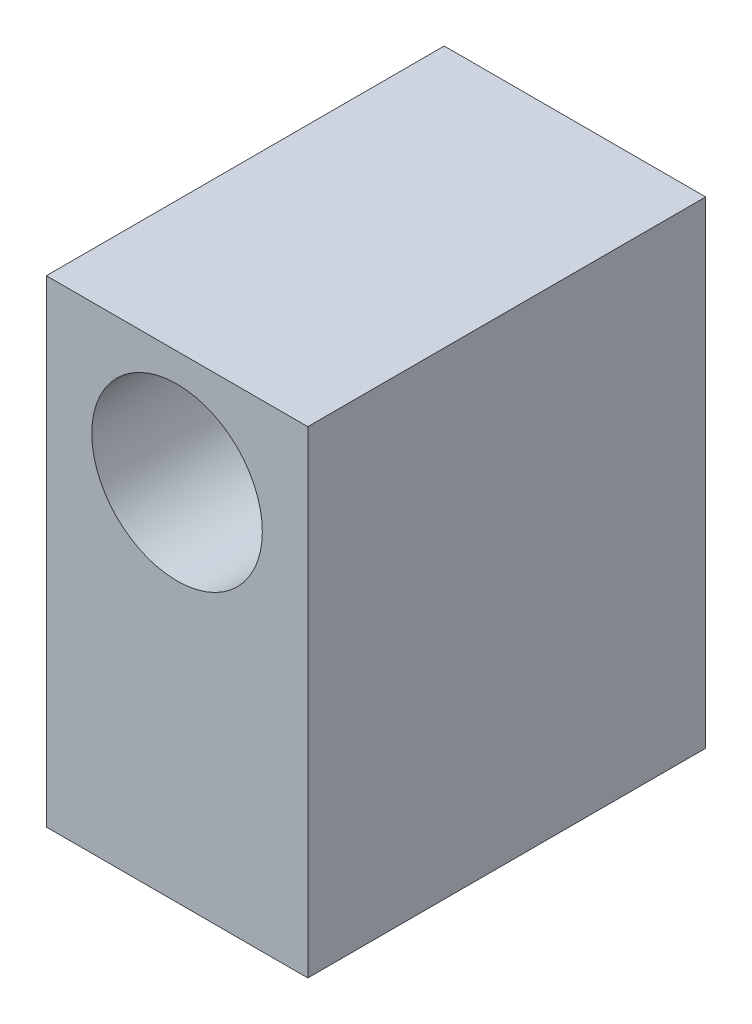
SolidWorks part; units mm, degrees
material "6061 合金"
ref_plane "前视基准面" through (0, 0, 0) normal (0, 0, 1) x (1, 0, 0)
ref_plane "上视基准面" through (0, 0, 0) normal (0, 1, 0) x (1, 0, 0)
ref_plane "右视基准面" through (0, 0, 0) normal (1, 0, 0) x (0, 0, -1)
sketch "草图1" plane through (0, 0, 0) normal (0, 0, 1) x (1, 0, 0)
  line L1 (-10.3871, 22.756) -> (12.6129, 22.756)
  line L2 (-10.3871, 22.756) -> (-10.3871, -19.244)
  line L3 (-10.3871, -19.244) -> (12.6129, -19.244)
  line L4 (12.6129, 22.756) -> (12.6129, -19.244)
  circle A0 centre (1.1129, 12.756) radius 7.5
  dimension "D3" = 15
  dimension "D1" = 23
  dimension "D2" = 42
  dimension "D4" = 11.5
  dimension "D5" = 10
extrude "凸台-拉伸1" add sketch "草图1" along normal blind 35
sketch "草图2" plane through (0, -19.244, 0) normal (0, -1, 0) x (1, 0, 0)
  line L0 (12.6129, 35) -> (12.6129, 0) construction
  line L1 (-10.3871, 35) -> (12.6129, 35) construction
  line L2 (-10.3871, 0) -> (12.6129, 0) construction
  circle A0 centre (1.1129, 27) radius 2.1
  circle A1 centre (1.1129, 8) radius 2.1
  dimension "D3" = 4.2
  dimension "D4" = 4.2
  dimension "D5" = 11.5
  dimension "D1" = 11.5
  dimension "D2" = 8
  dimension "D6" = 8
extrude "切除-拉伸1" cut sketch "草图2" against normal blind 11.5
sketch "草图3" plane through (0, -19.244, 0) normal (0, -1, 0) x (1, 0, 0)
  circle A0 centre (1.1129, 27) radius 2.5
  circle A1 centre (1.1129, 8) radius 2.5
  dimension "D1" = 5
  dimension "D2" = 5
extrude "切除-拉伸2" cut sketch "草图3" against normal blind 10
